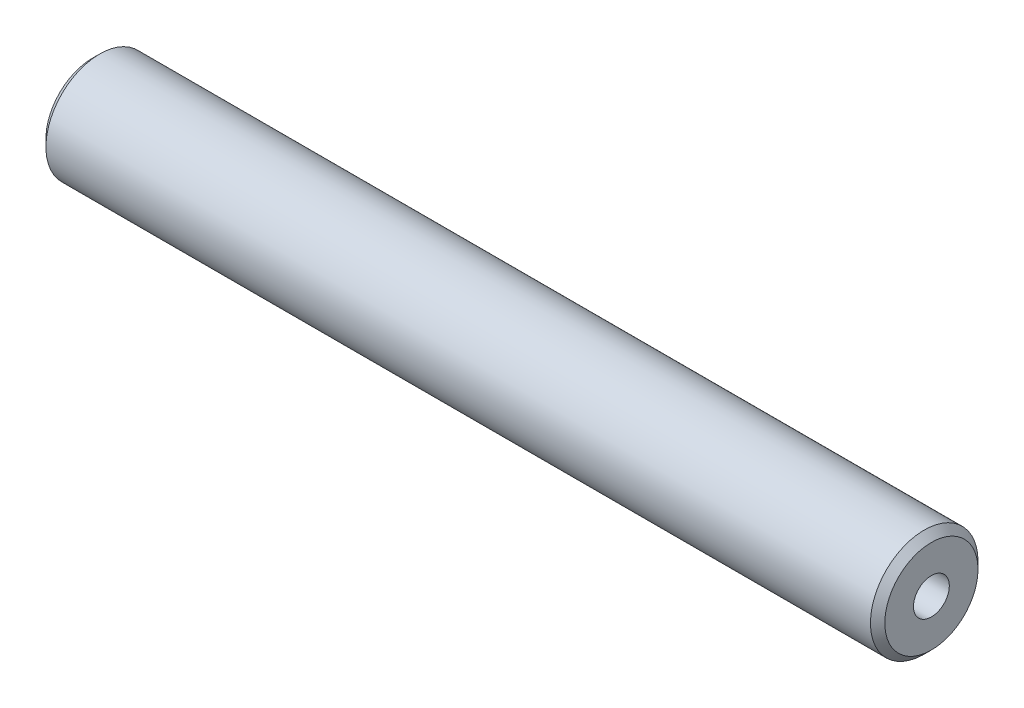
from build123d import *

# Parameters (mm, degrees)
SKETCH_1_R             = 7.5
EXTRUDE_1_DEPTH        = 117
HOLE_WIZARD_M4_1_D     = 3.3
HOLE_WIZARD_M4_1_DEPTH = 10.1
HOLE_WIZARD_M4_1_TIP   = 0.991420021
HOLE_WIZARD_M6_1_D     = 5
HOLE_WIZARD_M6_1_DEPTH = 15
HOLE_WIZARD_M6_1_TIP   = 1.502151548
CHAMFER_1_SIZE         = 1


with BuildPart() as part:
    # 草图1 → 凸台-拉伸1 (new body)
    with BuildSketch(Plane(origin=(0, 0, 0), x_dir=(0, 0, -1), z_dir=(1, 0, 0))):
        Circle(SKETCH_1_R)
    extrude(amount=EXTRUDE_1_DEPTH)

    # M4 螺纹孔1
    with Locations(Plane.ZY):
        with Locations((0, 0)):
            Hole(HOLE_WIZARD_M4_1_D / 2, depth=HOLE_WIZARD_M4_1_DEPTH)
            with Locations((0, 0, -(HOLE_WIZARD_M4_1_DEPTH + HOLE_WIZARD_M4_1_TIP / 2))):  # 118° drill point
                Cone(0, HOLE_WIZARD_M4_1_D / 2, HOLE_WIZARD_M4_1_TIP, mode=Mode.SUBTRACT)

    # M6 螺纹孔1
    with Locations(Plane(origin=(117, 0, 0), x_dir=(0, 0, -1), z_dir=(1, 0, 0))):
        with Locations((0, 0)):
            Hole(HOLE_WIZARD_M6_1_D / 2, depth=HOLE_WIZARD_M6_1_DEPTH)
            with Locations((0, 0, -(HOLE_WIZARD_M6_1_DEPTH + HOLE_WIZARD_M6_1_TIP / 2))):  # 118° drill point
                Cone(0, HOLE_WIZARD_M6_1_D / 2, HOLE_WIZARD_M6_1_TIP, mode=Mode.SUBTRACT)

    # 倒角1
    chamfer_1_edges = [part.edges().sort_by_distance(p)[0] for p in [
        (0, 0, 7.5),
        (117, 0, 7.5),
    ]]
    chamfer(chamfer_1_edges, length=CHAMFER_1_SIZE)


solid = part.part
